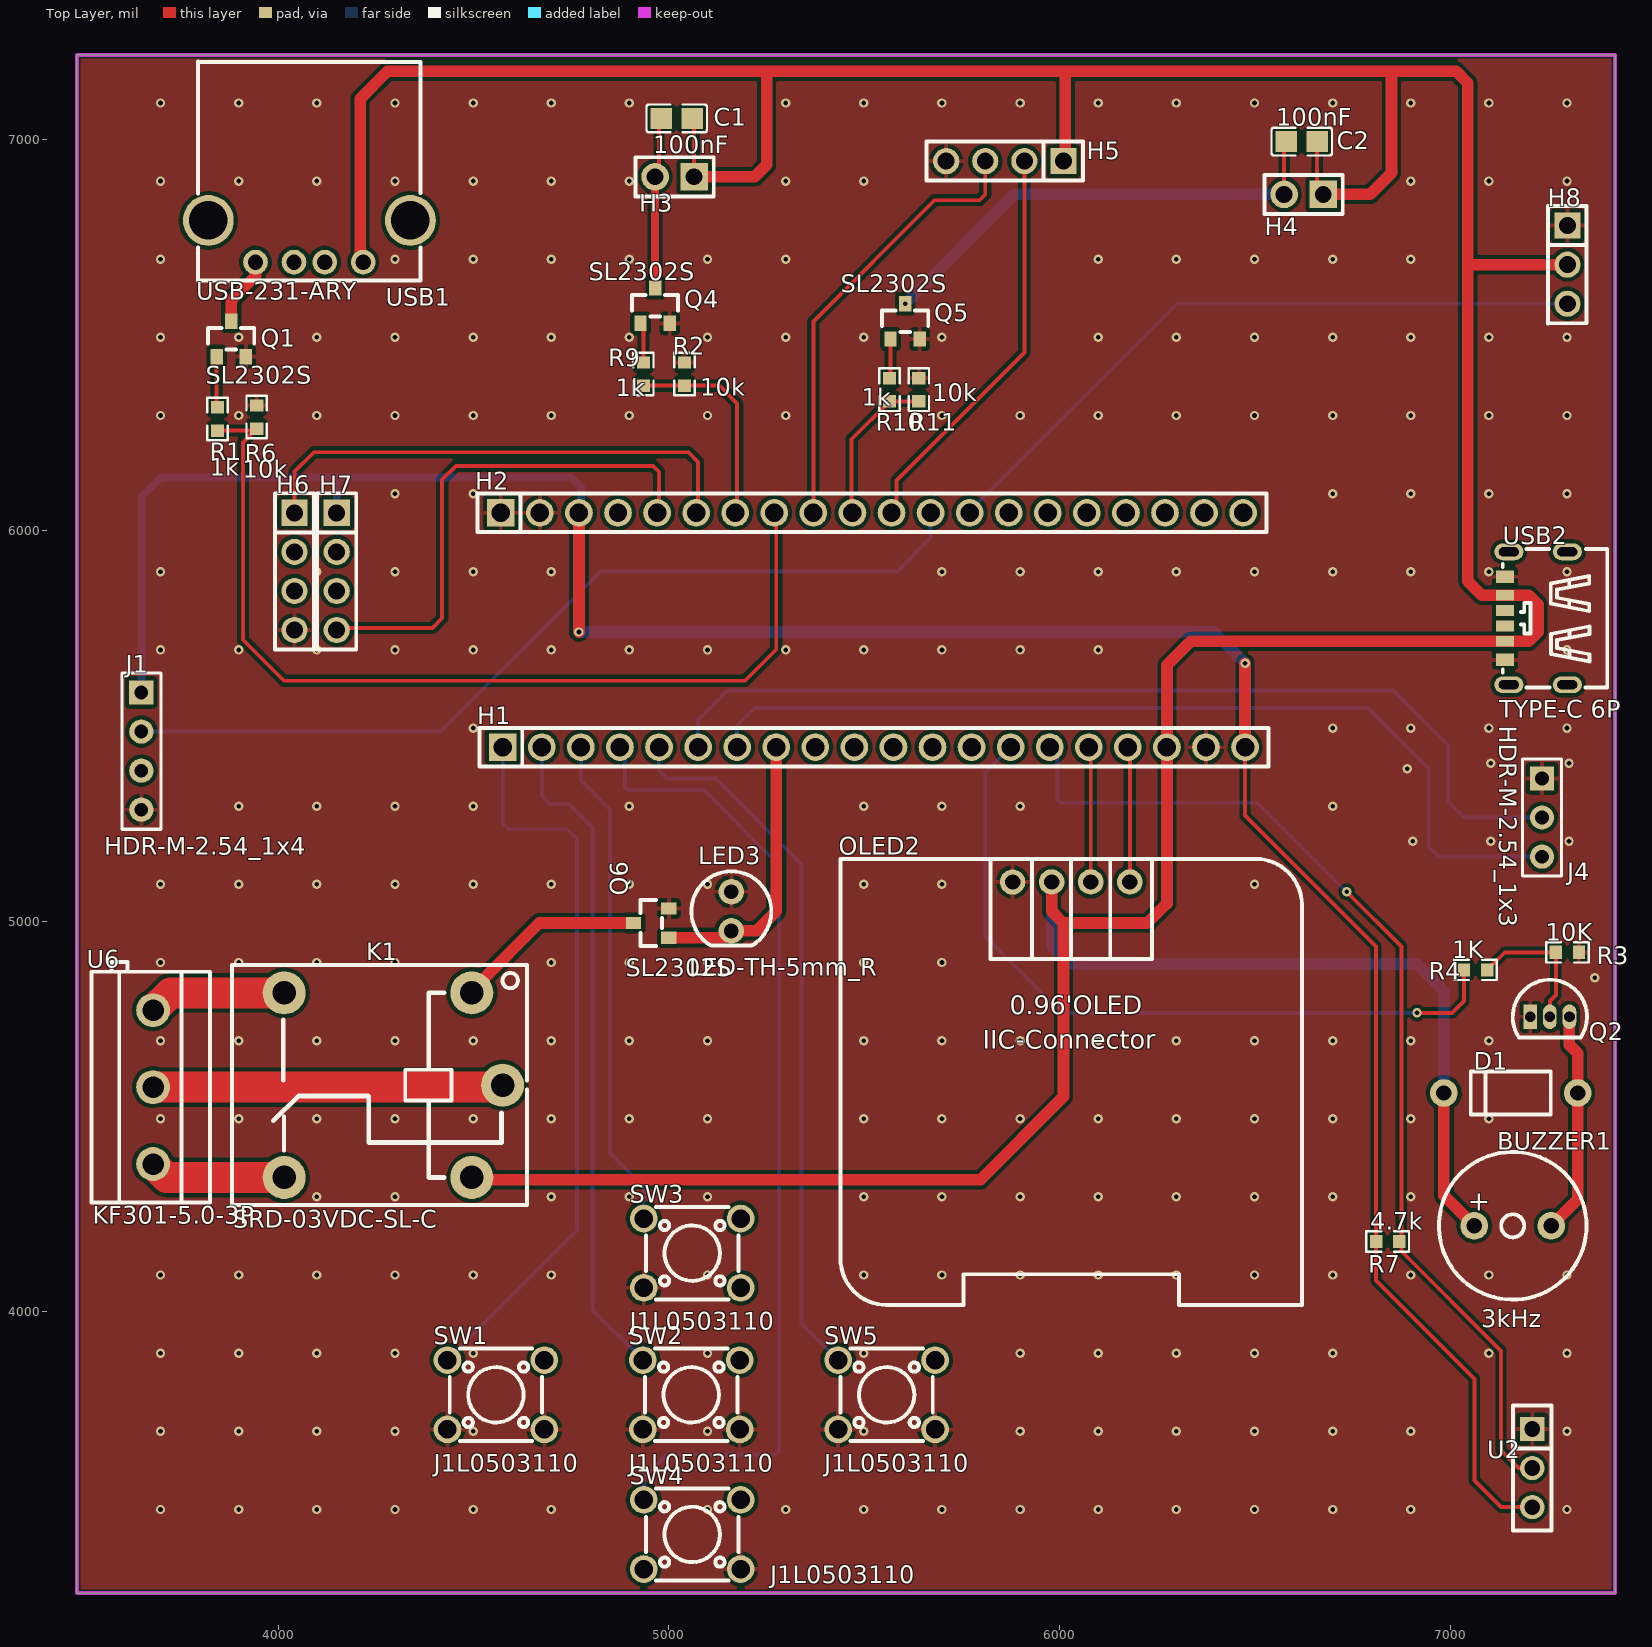
[diagram p0: Top Layer view]
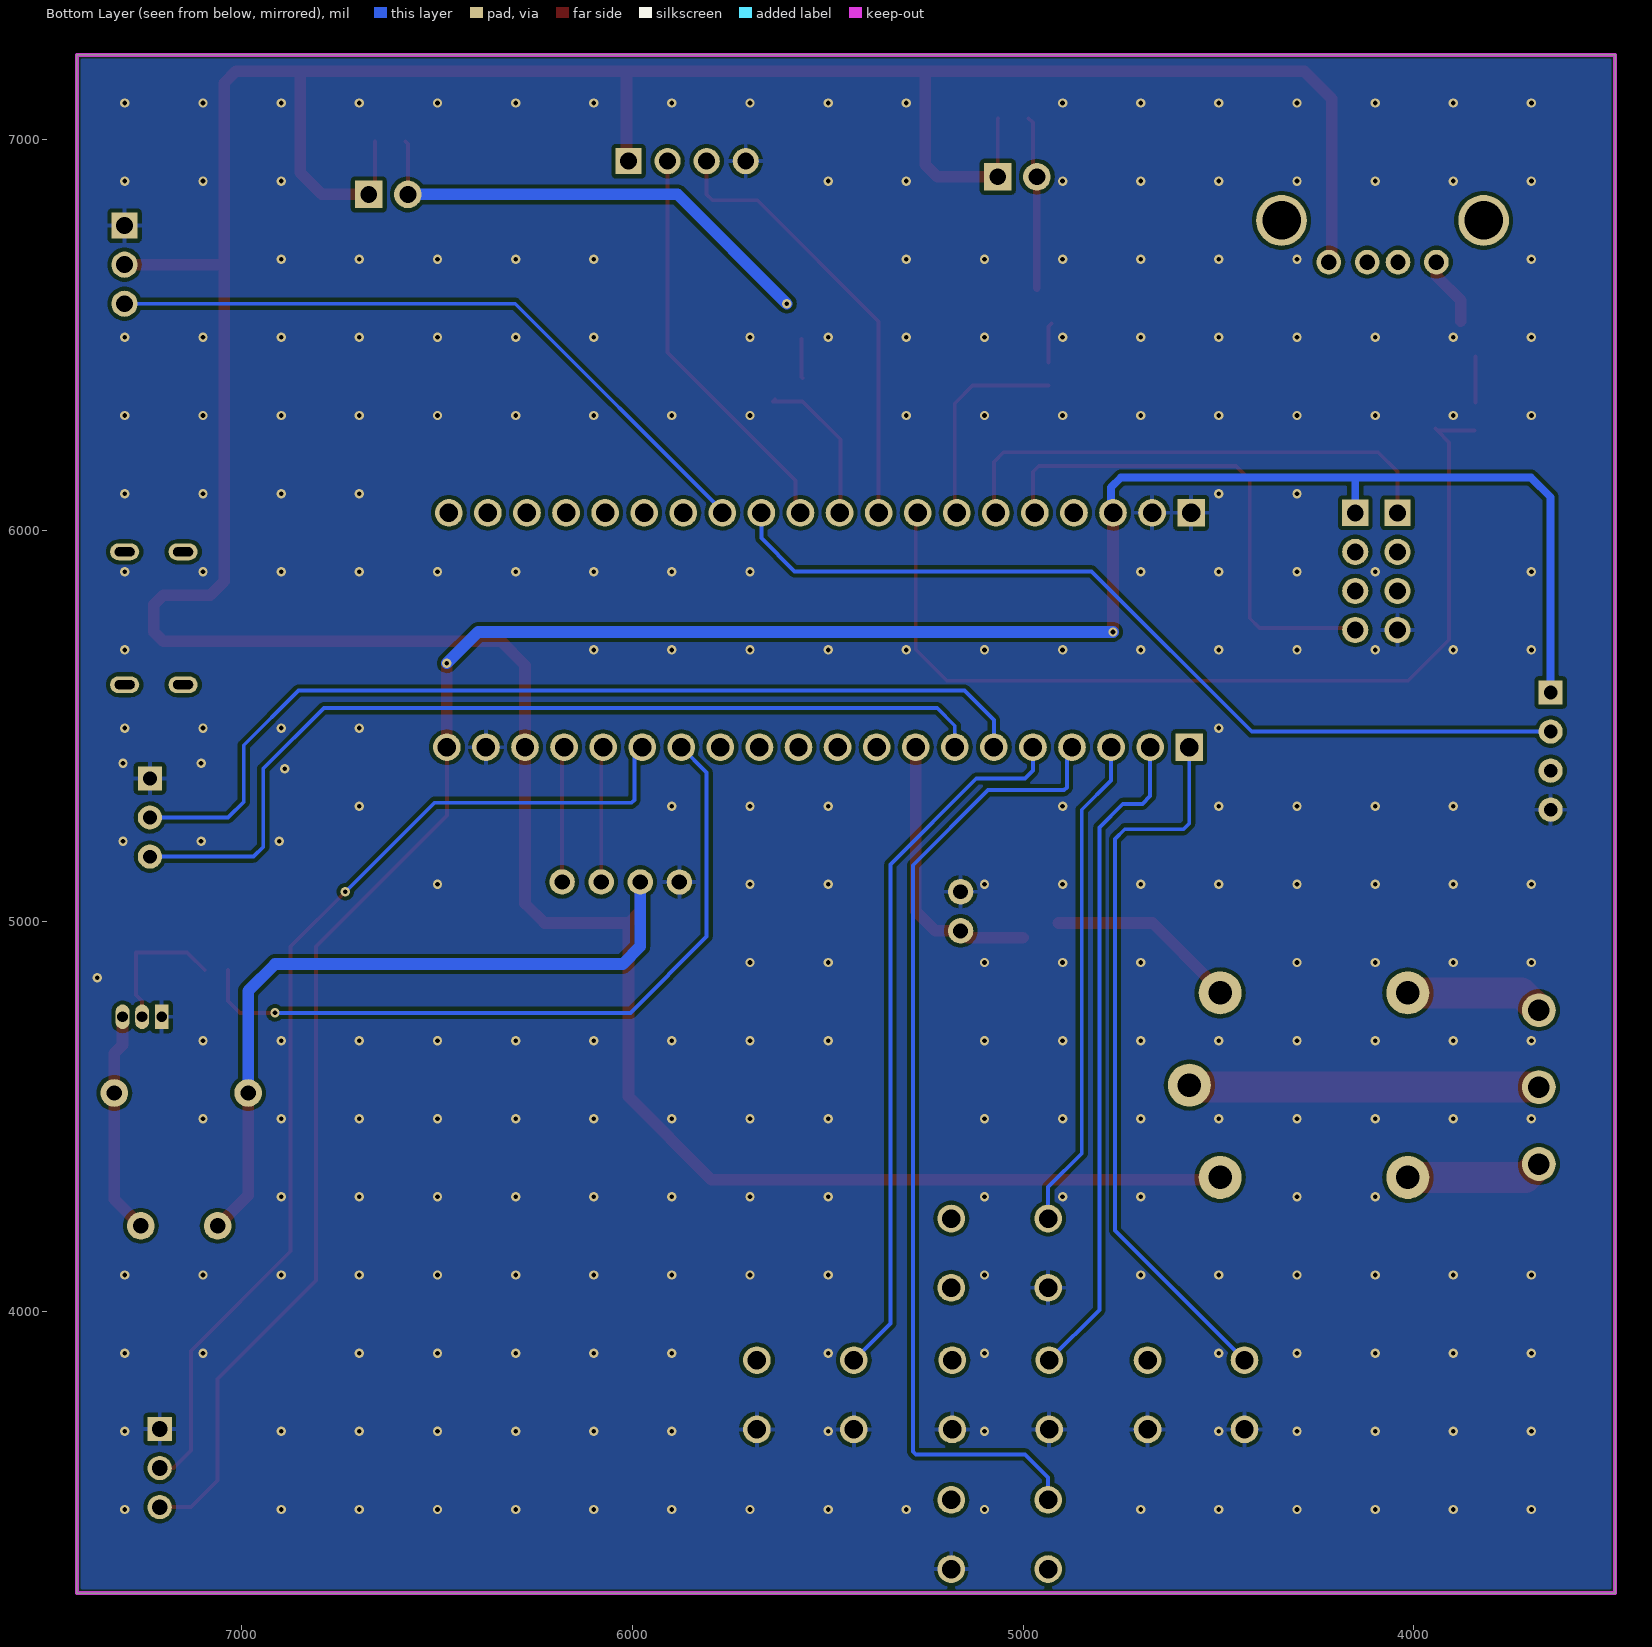
[diagram p1: Bottom Layer view, seen from below]
# Altium PCB MISC75408.pcbdoc
Units mil, origin at the board's own origin, x right, y up, seen from the top; angles counter-clockwise.
Board outline 3937 x 3937.11 mil, 2 copper layers (Top Layer, Bottom Layer), stack 62.206 mil thick; 40 components, 37 nets, 160 pads, 267 vias.

## Layer stack, top to bottom
Top Solder Mask Layer: solder mask 0.394, Dk 3.3
Top Layer: signal copper 1.379
Dielectric1: surface 59.449, FR4, Dk 4.5
Bottom Layer: signal copper 1.378
Bottom Solder Mask Layer: solder mask 0.394, Dk 3.3

## Board outline
3485,7217.01 3485,3279.9 7422,3279.9 7422,7217.01

## Design rules (kind name [scope] priority, off if disabled: settings)
BoardOutlineClearance copperThickness2oz_1 [All] p2 off: genericclearance=7.99 ignorepadtopadclearanceinfootprint=FALSE except(0: Arc-SplitContinuation Track-SplitContinuation SMDPad-SplitContinuation THPad-SplitContinuation Via-SplitContinuation Fill-SplitContinuation Region-SplitContinuation Poly-SplitContinuation Text-SplitContinuation Hole-SplitContinuation; 5.98: Arc-CutoutEdge SMDPad-CutoutEdge THPad-CutoutEdge Via-CutoutEdge Fill-CutoutEdge Region-CutoutEdge Text-CutoutEdge; 6.93: Hole-OutlineEdge Hole-CutoutEdge; 10: Poly-OutlineEdge Poly-CutoutEdge; 11.81: Arc-OutlineEdge Track-OutlineEdge SMDPad-OutlineEdge THPad-OutlineEdge Via-OutlineEdge Fill-OutlineEdge Region-OutlineEdge Text-OutlineEdge Track-CutoutEdge)
BoardOutlineClearance Plane_innerPlane_1 [All] p4 off: genericclearance=4.02 ignorepadtopadclearanceinfootprint=FALSE except(0: Arc-SplitContinuation Track-SplitContinuation SMDPad-SplitContinuation THPad-SplitContinuation Via-SplitContinuation Fill-SplitContinuation Region-SplitContinuation Poly-SplitContinuation Text-SplitContinuation Hole-SplitContinuation; 6: SMDPad-CutoutEdge THPad-CutoutEdge Via-CutoutEdge Fill-CutoutEdge Region-CutoutEdge Text-CutoutEdge; 6.93: Hole-OutlineEdge Hole-CutoutEdge; 10: Poly-OutlineEdge Poly-CutoutEdge; 11.8: Arc-OutlineEdge Track-OutlineEdge SMDPad-OutlineEdge THPad-OutlineEdge Via-OutlineEdge Fill-OutlineEdge Region-OutlineEdge Text-OutlineEdge; 11.81: Arc-CutoutEdge Track-CutoutEdge)
BoardOutlineClearance Copper_copperRegion_1 [All] p6 off: genericclearance=4.02 ignorepadtopadclearanceinfootprint=FALSE except(0: Arc-SplitContinuation Track-SplitContinuation SMDPad-SplitContinuation THPad-SplitContinuation Via-SplitContinuation Fill-SplitContinuation Region-SplitContinuation Poly-SplitContinuation Text-SplitContinuation Hole-SplitContinuation; 6: SMDPad-CutoutEdge THPad-CutoutEdge Via-CutoutEdge Fill-CutoutEdge Region-CutoutEdge Text-CutoutEdge; 6.93: Hole-OutlineEdge Hole-CutoutEdge; 10: Poly-OutlineEdge Poly-CutoutEdge; 11.8: Arc-OutlineEdge Track-OutlineEdge SMDPad-OutlineEdge THPad-OutlineEdge Via-OutlineEdge Fill-OutlineEdge Region-OutlineEdge Text-OutlineEdge; 11.81: Arc-CutoutEdge Track-CutoutEdge)
BoardOutlineClearance Copper_copperRegion_copperThickness1oz_1 [All] p8 off: genericclearance=4.02 ignorepadtopadclearanceinfootprint=FALSE except(0: Arc-SplitContinuation Track-SplitContinuation SMDPad-SplitContinuation THPad-SplitContinuation Via-SplitContinuation Fill-SplitContinuation Region-SplitContinuation Poly-SplitContinuation Text-SplitContinuation Hole-SplitContinuation; 6: SMDPad-CutoutEdge THPad-CutoutEdge Via-CutoutEdge Fill-CutoutEdge Region-CutoutEdge Text-CutoutEdge; 6.93: Hole-OutlineEdge Hole-CutoutEdge; 10: Poly-OutlineEdge Poly-CutoutEdge; 11.8: Arc-OutlineEdge Track-OutlineEdge SMDPad-OutlineEdge THPad-OutlineEdge Via-OutlineEdge Fill-OutlineEdge Region-OutlineEdge Text-OutlineEdge; 11.81: Arc-CutoutEdge Track-CutoutEdge)
BoardOutlineClearance Copper_copperRegion_Copper_copperRegion_1 [All] p10 off: genericclearance=4.02 ignorepadtopadclearanceinfootprint=FALSE except(0: Arc-SplitContinuation Track-SplitContinuation SMDPad-SplitContinuation THPad-SplitContinuation Via-SplitContinuation Fill-SplitContinuation Region-SplitContinuation Poly-SplitContinuation Text-SplitContinuation Hole-SplitContinuation; 6: SMDPad-CutoutEdge THPad-CutoutEdge Via-CutoutEdge Fill-CutoutEdge Region-CutoutEdge Text-CutoutEdge; 6.93: Hole-OutlineEdge Hole-CutoutEdge; 10: Poly-OutlineEdge Poly-CutoutEdge; 11.8: Arc-OutlineEdge Track-OutlineEdge SMDPad-OutlineEdge THPad-OutlineEdge Via-OutlineEdge Fill-OutlineEdge Region-OutlineEdge Text-OutlineEdge; 11.81: Arc-CutoutEdge Track-CutoutEdge)
BoardOutlineClearance copperThickness1oz_1 [All] p12: genericclearance=4.02 ignorepadtopadclearanceinfootprint=FALSE except(0: Arc-SplitContinuation Track-SplitContinuation SMDPad-SplitContinuation THPad-SplitContinuation Via-SplitContinuation Fill-SplitContinuation Region-SplitContinuation Poly-SplitContinuation Text-SplitContinuation Hole-SplitContinuation; 6: SMDPad-CutoutEdge THPad-CutoutEdge Via-CutoutEdge Fill-CutoutEdge Region-CutoutEdge Text-CutoutEdge; 6.93: Hole-OutlineEdge Hole-CutoutEdge; 10: Poly-OutlineEdge Poly-CutoutEdge; 11.8: Arc-OutlineEdge Track-OutlineEdge SMDPad-OutlineEdge THPad-OutlineEdge Via-OutlineEdge Fill-OutlineEdge Region-OutlineEdge Text-OutlineEdge; 11.81: Arc-CutoutEdge Track-CutoutEdge)
Clearance copperThickness2oz [All] p1 off: gap=7.99 ignorepadtopadclearanceinfootprint=FALSE except(5.98: SMDPad-Track SMDPad-SMDPad THPad-Track SMDPad-THPad THPad-THPad Track-Via SMDPad-Via THPad-Via Via-Via Fill-Track Region-Track Fill-SMDPad Region-SMDPad Fill-THPad Region-THPad Fill-Via Region-Via Fill-Fill Fill-Region Region-Region Arc-Track Arc-SMDPad Arc-THPad Arc-Via Fill-Arc Region-Arc Arc-Arc Text-Track SMDPad-Text Text-THPad Text-Via Fill-Text Region-Text Arc-Text Text-Text; 6.93: Hole-Track Hole-SMDPad Hole-THPad Hole-Via Fill-Hole Region-Hole Hole-Arc Hole-Text; 10: Poly-Track Poly-SMDPad Poly-THPad Poly-Via Poly-Fill Poly-Region Poly-Poly Poly-Arc Poly-Text Poly-Hole)
Clearance Plane_innerPlane [All] p3 off: gap=4.02 ignorepadtopadclearanceinfootprint=FALSE except(5.98: SMDPad-Track SMDPad-SMDPad THPad-Track SMDPad-THPad THPad-THPad Track-Via SMDPad-Via THPad-Via Via-Via Fill-Track Region-Track Fill-SMDPad Region-SMDPad Fill-THPad Region-THPad Fill-Via Region-Via Fill-Fill Fill-Region Region-Region; 6: Arc-Track Arc-SMDPad Arc-THPad Arc-Via Fill-Arc Region-Arc Arc-Arc Text-Track SMDPad-Text Text-THPad Text-Via Fill-Text Region-Text Arc-Text Text-Text; 6.93: Hole-Track Hole-SMDPad Hole-THPad Hole-Via Fill-Hole Region-Hole Hole-Arc Hole-Text; 10: Poly-Track Poly-SMDPad Poly-THPad Poly-Via Poly-Fill Poly-Region Poly-Poly Poly-Arc Poly-Text Poly-Hole)
Clearance Copper_copperRegion [All] p5 off: gap=4.02 ignorepadtopadclearanceinfootprint=FALSE except(5.98: SMDPad-Track SMDPad-SMDPad THPad-Track SMDPad-THPad THPad-THPad Track-Via SMDPad-Via THPad-Via Via-Via Fill-Track Region-Track Fill-SMDPad Region-SMDPad Fill-THPad Region-THPad Fill-Via Region-Via Fill-Fill Fill-Region Region-Region; 6: Arc-Track Arc-SMDPad Arc-THPad Arc-Via Fill-Arc Region-Arc Arc-Arc Text-Track SMDPad-Text Text-THPad Text-Via Fill-Text Region-Text Arc-Text Text-Text; 6.93: Hole-Track Hole-SMDPad Hole-THPad Hole-Via Fill-Hole Region-Hole Hole-Arc Hole-Text; 10: Poly-Track Poly-SMDPad Poly-THPad Poly-Via Poly-Fill Poly-Region Poly-Poly Poly-Arc Poly-Text Poly-Hole)
Clearance Copper_copperRegion_copperThickness1oz [All] p7 off: gap=4.02 ignorepadtopadclearanceinfootprint=FALSE except(5.98: SMDPad-Track SMDPad-SMDPad THPad-Track SMDPad-THPad THPad-THPad Track-Via SMDPad-Via THPad-Via Via-Via Fill-Track Region-Track Fill-SMDPad Region-SMDPad Fill-THPad Region-THPad Fill-Via Region-Via Fill-Fill Fill-Region Region-Region; 6: Arc-Track Arc-SMDPad Arc-THPad Arc-Via Fill-Arc Region-Arc Arc-Arc Text-Track SMDPad-Text Text-THPad Text-Via Fill-Text Region-Text Arc-Text Text-Text; 6.93: Hole-Track Hole-SMDPad Hole-THPad Hole-Via Fill-Hole Region-Hole Hole-Arc Hole-Text; 10: Poly-Track Poly-SMDPad Poly-THPad Poly-Via Poly-Fill Poly-Region Poly-Poly Poly-Arc Poly-Text Poly-Hole)
Clearance Copper_copperRegion_Copper_copperRegion [All] p9 off: gap=4.02 ignorepadtopadclearanceinfootprint=FALSE except(5.98: SMDPad-Track SMDPad-SMDPad THPad-Track SMDPad-THPad THPad-THPad Track-Via SMDPad-Via THPad-Via Via-Via Fill-Track Region-Track Fill-SMDPad Region-SMDPad Fill-THPad Region-THPad Fill-Via Region-Via Fill-Fill Fill-Region Region-Region; 6: Arc-Track Arc-SMDPad Arc-THPad Arc-Via Fill-Arc Region-Arc Arc-Arc Text-Track SMDPad-Text Text-THPad Text-Via Fill-Text Region-Text Arc-Text Text-Text; 6.93: Hole-Track Hole-SMDPad Hole-THPad Hole-Via Fill-Hole Region-Hole Hole-Arc Hole-Text; 10: Poly-Track Poly-SMDPad Poly-THPad Poly-Via Poly-Fill Poly-Region Poly-Poly Poly-Arc Poly-Text Poly-Hole)
Clearance copperThickness1oz [All] p11: gap=4.02 ignorepadtopadclearanceinfootprint=FALSE except(5.98: SMDPad-Track SMDPad-SMDPad THPad-Track SMDPad-THPad THPad-THPad Track-Via SMDPad-Via THPad-Via Via-Via Fill-Track Region-Track Fill-SMDPad Region-SMDPad Fill-THPad Region-THPad Fill-Via Region-Via Fill-Fill Fill-Region Region-Region; 6: Arc-Track Arc-SMDPad Arc-THPad Arc-Via Fill-Arc Region-Arc Arc-Arc Text-Track SMDPad-Text Text-THPad Text-Via Fill-Text Region-Text Arc-Text Text-Text; 6.93: Hole-Track Hole-SMDPad Hole-THPad Hole-Via Fill-Hole Region-Hole Hole-Arc Hole-Text; 10: Poly-Track Poly-SMDPad Poly-THPad Poly-Via Poly-Fill Poly-Region Poly-Poly Poly-Arc Poly-Text Poly-Hole)
DiffPairsRouting differentialPair [All] p1: maxlimit=6 minlimit=6 mostfreqgap=6 toplayer_minwidth=5 toplayer_prefwidth=10 toplayer_maxwidth=100 toplayer_mingap=6 toplayer_prefgap=6 toplayer_maxgap=6 bottomlayer_minwidth=5 bottomlayer_prefwidth=10 bottomlayer_maxwidth=100 bottomlayer_mingap=6 bottomlayer_prefgap=6 bottomlayer_maxgap=6 maxuncoupledlength=10
HoleToHoleClearance otherClearance [All] p1: gap=11.81 allowstackedmicrovias=TRUE
Length netLength [All] p1: minlimit=0 maxlimit=0
PasteMaskExpansion pasteMaskExpansion [All] p1: expansion=0
PlaneConnect innerPlane [All] p1: planeconnectstyle=Relief reliefexpansion=20 reliefentries=4 reliefconductorwidth=10 reliefairgap=10
PolygonConnect copperRegion_copperThickness1oz [All] p1 off: connectstyle=Relief reliefconductorwidth=10 reliefentries=4 polygonreliefangle="90 Angle" airgapwidth=10 via.connectstyle=Relief via.reliefconductorwidth=10 via.reliefentries=4 via.polygonreliefangle="90 Angle" via.airgapwidth=10
PolygonConnect copperRegion_Copper_copperRegion [All] p2 off: connectstyle=Relief reliefconductorwidth=10 reliefentries=4 polygonreliefangle="90 Angle" airgapwidth=10 via.connectstyle=Relief via.reliefconductorwidth=10 via.reliefentries=4 via.polygonreliefangle="90 Angle" via.airgapwidth=10
PolygonConnect copperRegion [All] p3: connectstyle=Relief reliefconductorwidth=10 reliefentries=4 polygonreliefangle="90 Angle" airgapwidth=10 via.connectstyle=Relief via.reliefconductorwidth=10 via.reliefentries=4 via.polygonreliefangle="90 Angle" via.airgapwidth=10
RoutingVias viaSize [All] p1: holewidth=12.01 width=24.02 viastyle="Through Hole" minholewidth=11.81 minwidth=19.68 maxholewidth=248.03 maxwidth=393.7
SolderMaskExpansion solderMaskExpansion [IsVia] p1: expansion=-1000 istentingtop=TRUE
SolderMaskExpansion solderMaskExpansion [All] p2: expansion=2 istentingtop=FALSE
Width copperThickness2oz_2 [All] p1 off: maxlimit=100 minlimit=8 preferedwidth=10
Width copperThickness1oz_2 [All] p2: maxlimit=100 minlimit=5 preferedwidth=10

## Components (designator, comment, footprint, x,y, rotation, side; value= is the part's Value field where it differs from the comment)
BUZZER1 "3kHz" BUZ-TH_BD9.6-P5.00-D0.7-FD 7160,4220 r0 top
C1 "100nF" C0805 5020.31,7054.47 r180 top
C2 "100nF" C0805 6620,6995 r180 top
D1 "" DO_1N4007 7155,4560 r0 top
H1 "" HDR-TH_20P-P2.54-V-F 5525,5445 r0 top
H2 "" HDR-TH_20P-P2.54-V-F 5520,6045 r0 top
H3 "" HDR-TH_2P-P2.54-V-M-1 5015,6905 r180 top
H4 "" HDR-TH_2P-P2.54-V-M-1 6625,6860 r180 top
H5 "" HDR-TH_4P-P2.54-V-M 5860,6945 r180 top
H6 "" HDR-TH_4P-P2.54-V-M 4041.84,5895 r270 top
H7 "" HDR-TH_4P-P2.54-V-M 4150,5895 r270 top
H8 "" HDR-TH_3P-P2.54-V-M 7300,6680 r270 top
J1 "HDR-M-2.54_1x4" HDR-M-2.54_1X4 3650,5435 r270 top
J4 "HDR-M-2.54_1x3" HDR-M-2.54_1X3 7235,5265 r270 top
K1 "SRD-03VDC-SL-C" RELAY-TH_SRD-XXVDC-XL-C 4295,4580 r180 top
LED3 "LED-TH-5mm_R" LED-TH_BD5.0_RED 5160,5025 r0 top
OLED2 "" 0.96OLED_4P 6030,5100 r0 top
Q1 "SL2302S" SOT-23_L2.9-W1.3-P1.90-LS2.4-BR 3880,6490 r270 top
Q2 "" S8050_TO_92 7255,4755 r0 top
Q4 "SL2302S" SOT-23_L2.9-W1.3-P1.90-LS2.4-BR 4965,6575 r270 top
Q5 "SL2302S" SOT-23_L2.9-W1.3-P1.90-LS2.4-BR 5605,6535 r270 top
Q6 "SL2302S" SOT-23_L2.9-W1.3-P1.90-LS2.4-BR 4955,4995 r0 top
R1 "1k" R0603 3845,6285 r90 top
R2 "10k" R0603 5040,6400 r90 top
R3 "10K" R0603 7300,4920 r180 top
R4 "1K" R0603 7065,4875 r180 top
R6 "10k" R0603 3945,6290 r90 top
R7 "4.7k" R0603 6840,4180 r180 top
R9 "1k" R0603 4935,6400 r90 top
R10 "1k" R0603 5565,6360 r90 top
R11 "10k" R0603 5640,6360 r90 top
SW1 "J1L0503110" SW-TH_4P-L6.0-W6.0-P4.50-LS6.3 4557.5,3787.5 r0 top
SW2 "J1L0503110" SW-TH_4P-L6.0-W6.0-P4.50-LS6.3 5057.5,3787.5 r0 top
SW3 "J1L0503110" SW-TH_4P-L6.0-W6.0-P4.50-LS6.3 5060,4150 r0 top
SW4 "J1L0503110" SW-TH_4P-L6.0-W6.0-P4.50-LS6.3 5060,3430 r0 top
SW5 "J1L0503110" SW-TH_4P-L6.0-W6.0-P4.50-LS6.3 5557.5,3787.5 r0 top
U2 "DS18B20+" HDR-TH_3P-P2.54-V-F 7210,3600 r270 top
U6 "KF301-5.0-3P" CONN-TH_3P-P5.00_KF301-5.0-3P 3680,4575 r90 top
USB1 "USB-231-ARY" USB-A-TH_USB-231-ARY 4080,6740 r180 top
USB2 "TYPE-C 6P" TYPE-C-SMD_TYPE-C-6P_1 7220,5775 r90 top

## Footprints (in the part's own frame and the unit in brackets; to place one, negate y for a bottom-side part, rotate by r counter-clockwise, add the part's x,y. Pads: shape width x height; smd on the part's side, far side on the other; paste and mask are expansions set on the pad)
0.96OLED_4P [mm]
  round 1.65 hole 1 copper offset 0,0: 1(-3.81,-0.001) 2(-1.27,0.002) 3(1.27,0.002) 4(3.81,0.002)
  silkscreen extent -15,-27.5 15,1.5
BUZ-TH_BD9.6-P5.00-D0.7-FD [mm]
  round 1.8 hole 1: 1(-2.5,0) 2(2.5,0)
  silkscreen extent -4.8,-4.8 4.8,4.8
C0805 [mm]
  rect 1.41x1.35 smd paste-100 mask+0.051: 1(-1,0) 2(1,0)
  silkscreen extent -1.96,-0.9 1.96,0.9
CONN-TH_3P-P5.00_KF301-5.0-3P [mm]
  round 2.2 hole 1.4 paste+0 mask+0.051: 1(-5,0) 2(0,0) 3(5,0)
  silkscreen extent -7.5,-3.7 8.13,4
DO_1N4007 [mm]
  round 1.8 hole 1 paste+0 mask+0.051: 1(-4.35,0) 2(4.35,0)
  silkscreen extent -2.6,-1.4 2.6,1.4
HDR-M-2.54_1X3 [mil]
  rect 62x62 hole 35 paste+0 mask+2: 1(-100,0)
  round 62 hole 35 paste+0 mask+2: 2(0,0) 3(100,0)
  silkscreen extent -150,-50 150,50
HDR-M-2.54_1X4 [mil]
  rect 62x62 hole 35 paste+0 mask+2: 1(-150,0)
  round 62 hole 35 paste+0 mask+2: 2(-50,0) 3(50,0) 4(150,0)
  silkscreen extent -200,-50 200,50
HDR-TH_2P-P2.54-V-M-1 [mm]
  rect 1.8x1.8 hole 1.1: 1(-1.27,0)
  round 1.8 hole 1.1: 2(1.27,0)
  silkscreen extent -2.54,-1.27 2.54,1.27
HDR-TH_3P-P2.54-V-F [mil]
  rect 62x62 hole 40.16: 1(-100,0)
  round 62 hole 40.16: 2(0,0) 3(100,0)
  silkscreen extent -160,-49 160,49
HDR-TH_3P-P2.54-V-M [mm]
  rect 1.7x1.7 hole 1.1: 1(-2.54,0)
  round 1.7 hole 1.1: 2(0,0) 3(2.54,0)
  silkscreen extent -3.81,-1.25 3.81,1.25
HDR-TH_4P-P2.54-V-M [mm]
  rect 1.7x1.7 hole 1.1: 1(-3.81,0)
  round 1.7 hole 1.1: 2(-1.27,0) 3(1.27,0) 4(3.81,0)
  silkscreen extent -5.08,-1.27 5.08,1.27
HDR-TH_20P-P2.54-V-F [mm]
  rect 1.8x1.8 hole 1.2: 1(-24.13,0)
  round 1.8 hole 1.2: 2(-21.59,0) 3(-19.05,0) 4(-16.51,0) 5(-13.97,0) 6(-11.43,0) 7(-8.89,0) 8(-6.35,0) 9(-3.81,0) 10(-1.27,0) 11(1.27,0) 12(3.81,0) 13(6.35,0) 14(8.89,0) 15(11.43,0) 16(13.97,0) 17(16.51,0) 18(19.05,0) 19(21.59,0) 20(24.13,0)
  silkscreen extent -25.65,-1.25 25.65,1.25
LED-TH_BD5.0_RED [mil]
  round 65 hole 38 paste+0 mask+2: 1(0,50) 2(0,-50)
  silkscreen extent -102,-88 102,102
R0603 [mil]
  rect 31.75x34.02 smd paste-3937.01 mask+2: 1(-29.66,-0.01) 2(29.66,0.01)
  silkscreen extent -55,-26 55,26
RELAY-TH_SRD-XXVDC-XL-C [mil]
  round 110 hole 60 paste+0 mask+2: 1(-200.79,-236.22) 2(279.53,-236.2) 3(279.53,236.2) 4(-200.79,236.22) 5(-279.53,0)
  silkscreen extent -342,-307 413,307
S8050_TO_92 [mil]
  rect 35.4x63 hole 27.6 paste+0 mask+2: 1(-50,0)
  oval 35.4x63 hole 27.6 paste+0 mask+2: 2(0,0) 3(50,0)
  silkscreen extent -95,-53 95,95
SOT-23_L2.9-W1.3-P1.90-LS2.4-BR [mm]
  rect 1x0.8 smd paste+0 mask+0.051: 1(1.15,-0.95) 2(1.15,0.95) 3(-1.15,0)
  silkscreen extent -0.7,-1.5 0.7,1.5
SW-TH_4P-L6.0-W6.0-P4.50-LS6.3 [mm]
  round 1.8 hole 1.2: 1(-3.15,2.25) 2(3.15,2.25) 3(-3.15,-2.25) 4(3.15,-2.25)
  silkscreen extent -3,-3 3,3
TYPE-C-SMD_TYPE-C-6P_1 [mm]
  oval 1.1x1.9 hole 0.6 slot 1.3 at 90 deg paste+0 mask+0.051: 7(-4.32,1.775) 7(-4.32,-2.025) 7(4.32,1.775)
  oval 1.1x1.9 hole 0.6 slot 1.3 at 90 deg copper offset 0,0 paste+0 mask+0.051: 7(4.32,-2.025)
  rect 0.7x1.2 smd paste-100 mask+0.051: A5(-0.5,2.025) A9(1.5,2.025) B5(0.5,2.025) B9(-1.5,2.025)
  rect 0.8x1.2 smd paste-100 mask+0.051: A12(2.7,2.025) B12(-2.7,2.025)
  silkscreen extent -4.5,-4.63 4.5,2.18
USB-A-TH_USB-231-ARY [mm]
  round 1.6 hole 1: 1(-3.5,1.355) 2(-1,1.355) 3(1,1.355) 4(3.5,1.355)
  round 3.3 hole 2.5: 5(-6.57,-1.355) 6(6.57,-1.355)
  silkscreen extent -7.23,-11.68 7.24,2.54

## Via types
v1: diameter 24.02, hole 12, Top Layer to Bottom Layer, 267 vias

## Nets (pads, with @x,y where several pads share a name; then routed paths per layer and width w, separated by ;. In a path a pad name is that pad's centre, name@x,y a point inside that pad or via, vN(x,y) a via of type N, cw(c..) or ccw(c..) an arc to the next point about the centre after c; other vN are vias at no path point)
$1N2: Q1.3 USB1.4 | length 177.2
  Top Layer w30: Q1.3 3880,6588.86 3942.21,6651.07 USB1.4
$1N4: Q1.1 R1.2 | length 117
  Top Layer w10: R1.2@3842.6,6327.74 Q1.1
$1N10: BUZZER1.2 D1.2 Q2.3 | length 571.9
  Top Layer w30: BUZZER1.2 7326.26,4287.84 D1.2 7326.26,4661.65 7305,4682.91 Q2.3
$1N26: Q4.1 R9.2 | length 103.1
  Top Layer w10: Q4.1 4935,6522.32 R9.2
$1N27: C1.2 H3.2 Q4.3 | length 442.9
  Top Layer w10: H3.2 4975,6915 4975,7043.54 C1.2@4985.94,7054.47
  Top Layer w20: Q4.3 H3.2
$1N30: C2.2 H4.2 Q5.3 | length 1223.2
  Top Layer w10: H4.2 6575,6989.37 C2.2
  Bottom Layer w30: v1(5605,6580.27) 5884.73,6860 H4.2
$1N32: Q5.1 R10.2 | length 101.1
  Top Layer w10: R10.2 5567.6,6392.26 Q5.1
$1N35: K1.2 U6.3 | length 353.8
  Top Layer w80: U6.3 3724.35,4816.2 K1.2
$1N38: K1.5 U6.2 | length 896.6
  Top Layer w80: U6.2 4569.53,4575 K1.5
$1N39: K1.3 U6.1 | length 349.7
  Top Layer w80: U6.1 3714.35,4343.8 K1.3
$1N121: K1.1 Q6.3 | length 457.1
  Top Layer w30: K1.1@4515.89,4842.23 4668.66,4995 Q6.3
$1N124: Q2.2 R3.2 R4.1 | length 365.7
  Top Layer w10: R4.1 7139.66,4920 R3.2 7270.34,4810.34 7255,4795 Q2.2
+5V: BUZZER1.1 C1.1 C2.1 D1.1 H1.18 H3.1 H4.1 H5.1 H8.2 K1.4 OLED2.2 USB1.1 USB2.A9 USB2.B9 | length 12373.8
  Top Layer w10: C1.1@5064.68,7054.47 5065,7054.15 H3.1 ; C2.1 6659.37,6875.63 H4.1
  Top Layer w30: USB1.1 4210,6694.45 4210,7105 4280,7175 5250.56,7175 ; K1.4@4528.61,4337.87 5797.87,4337.87 6010,4550 6010,4995 ; H3.1 5220,6905 5250.56,6935.56 5250.56,7175 ; OLED2.2@5980,5100.05 5980,5025 6010,4995 ; H5.1@6015,6955 6015,7175 ; H4.1 6795,6860 6850,6915 6850,7173.29 6851.71,7175 ; D1.1 6983.74,4297.84 BUZZER1.1 ; H8.2 7049.06,6680 7045,6675.94 ; 5250.56,7175 6015,7175 ; 6010,4995 6225,4995 6275,5045 H1.18 6275,5655 6335.95,5715.95 7140.27,5715.95 7200.95,5715.95 7225,5740 7225,5810 7200.94,5834.06 USB2.A9 7080.94,5834.06 7045,5870 7045,6675.94 ; 6015,7175 6851.71,7175 ; 6851.71,7175 7015,7175 7045,7145 7045,6675.94
  Bottom Layer w30: OLED2.2@5980,5100.05 5980,4935 6025,4890 6915,4890 6983.74,4821.26 D1.1
GND: H1.19 H2.1 H2.2 H5.4 H6.4 H8.1 J1.4 J4.1 LED3.1 OLED2.1 Q1.2 Q2.1 Q4.2 Q5.2 Q6.2 R2.2 R3.1 R6.2 R11.2 SW1.3 SW1.4 SW2.3 SW2.4 SW3.3 SW4.4 SW5.3 SW5.4 U2.1 USB2.A12 USB2.B12
  other v1: 3699.1,3494 3899.1,3494 4099.1,3494 4299.1,3494 4499.1,3494 4699.1,3494 5099.1,3494 5299.1,3494 5499.1,3494 5699.1,3494 5899.1,3494 6099.1,3494 6299.1,3494 6499.1,3494 6699.1,3494 6899.1,3494 7299.1,3494 3699.1,3694 3899.1,3694 4099.1,3694 4299.1,3694 4499.1,3694 5099.1,3694 5499.1,3694 5899.1,3694 6099.1,3694 6299.1,3694 6499.1,3694 6699.1,3694 6899.1,3694 7299.1,3694 3699.1,3894 3899.1,3894 4099.1,3894 4299.1,3894 4499.1,3894 5099.1,3894 5499.1,3894 5899.1,3894 6099.1,3894 6299.1,3894 6499.1,3894 6699.1,3894 7099.1,3894 7299.1,3894 3699.1,4094 3899.1,4094 4099.1,4094 4299.1,4094 4499.1,4094 4699.1,4094 5099.1,4094 5499.1,4094 5699.1,4094 5899.1,4094 6099.1,4094 6299.1,4094 6499.1,4094 6699.1,4094 6899.1,4094 7099.1,4094 7299.1,4094 4099.1,4294 4299.1,4294 4699.1,4294 4899.1,4294 5099.1,4294 5499.1,4294 5699.1,4294 5899.1,4294 6099.1,4294 6299.1,4294 6499.1,4294 6699.1,4294 6899.1,4294 3699.1,4494 3899.1,4494 4099.1,4494 4299.1,4494 4499.1,4494 4699.1,4494 4899.1,4494 5099.1,4494 5499.1,4494 5699.1,4494 5899.1,4494 6099.1,4494 6299.1,4494 6499.1,4494 6699.1,4494 6899.1,4494 7099.1,4494 3699.1,4694 3899.1,4694 4099.1,4694 4299.1,4694 4499.1,4694 4699.1,4694 4899.1,4694 5099.1,4694 5499.1,4694 5699.1,4694 5899.1,4694 6099.1,4694 6299.1,4694 6499.1,4694 6699.1,4694 6899.1,4694 7099.1,4694 7370,4855 3699.1,4894 3899.1,4894 4099.1,4894 4299.1,4894 4699.1,4894 4899.1,4894 5099.1,4894 5499.1,4894 5699.1,4894 3699.1,5094 3899.1,5094 4099.1,5094 4299.1,5094 4499.1,5094 4699.1,5094 4899.1,5094 5099.1,5094 5499.1,5094 5699.1,5094 6499.1,5094 6904.1,5204 7104.1,5204 7304.1,5204 3899.1,5294 4099.1,5294 4299.1,5294 4499.1,5294 4899.1,5294 5499.1,5294 5699.1,5294 5899.1,5294 6699.1,5294 6890,5390 7104.1,5404 7304.1,5404 4499.1,5494 6699.1,5494 6899.1,5494 7099.1,5494 7299.1,5494 3699.1,5694 3899.1,5694 4099.1,5694 4299.1,5694 4499.1,5694 4699.1,5694 4899.1,5694 5099.1,5694 5299.1,5694 5499.1,5694 5699.1,5694 5899.1,5694 6099.1,5694 7299.1,5694 3699.1,5894 4099.1,5894 4299.1,5894 4499.1,5894 4699.1,5894 5699.1,5894 5899.1,5894 6099.1,5894 6299.1,5894 6499.1,5894 6699.1,5894 6899.1,5894 7099.1,5894 7299.1,5894 4299.1,6094 4499.1,6094 6699.1,6094 6899.1,6094 7099.1,6094 7299.1,6094 3699.1,6294 3899.1,6294 4099.1,6294 4299.1,6294 4499.1,6294 4699.1,6294 4899.1,6294 5099.1,6294 5299.1,6294 5699.1,6294 5899.1,6294 6099.1,6294 6299.1,6294 6499.1,6294 6699.1,6294 6899.1,6294 7099.1,6294 7299.1,6294 3699.1,6494 3899.1,6494 4099.1,6494 4299.1,6494 4499.1,6494 4699.1,6494 4899.1,6494 5099.1,6494 5299.1,6494 5499.1,6494 5699.1,6494 6099.1,6494 6299.1,6494 6499.1,6494 6699.1,6494 6899.1,6494 7099.1,6494 7299.1,6494 3699.1,6694 4299.1,6694 4499.1,6694 4699.1,6694 4899.1,6694 5099.1,6694 5299.1,6694 6099.1,6694 6299.1,6694 6499.1,6694 6699.1,6694 6899.1,6694 3699.1,6894 3899.1,6894 4099.1,6894 4299.1,6894 4499.1,6894 4699.1,6894 4899.1,6894 5299.1,6894 5499.1,6894 6899.1,6894 7099.1,6894 7299.1,6894 3699.1,7094 3899.1,7094 4099.1,7094 4299.1,7094 4499.1,7094 4699.1,7094 4899.1,7094 5299.1,7094 5499.1,7094 5699.1,7094 5899.1,7094 6099.1,7094 6299.1,7094 6499.1,7094 6699.1,7094 6899.1,7094 7099.1,7094 7299.1,7094
PA3: H2.13 H8.3 | length 1754.5
  Bottom Layer w10: H2.13 5770,6050 6300,6580 H8.3
PA4: H2.12 J1.2 | length 2290
  Bottom Layer w10: J1.2 4415,5485 4825,5895 5585,5895 5670,5980 H2.12
PA5: H2.11 H5.2 | length 1040.8
  Top Layer w10: H2.11 5582.93,6057.93 5582.93,6127.93 5910,6455 H5.2
PA6: H2.10 R10.1 R11.1 | length 410.5
  Top Layer w10: H2.10@5475,6045 5467.93,6052.07 5467.93,6233.27 R10.1 R11.1@5630,6330.34 ; R11.1@5635,6335.34 R11.1@5630,6330.34 ; R11.1 R11.1@5630,6330.34
PA7: H2.9 H5.3 | length 1149.6
  Top Layer w10: H2.9 5370,6535 5680,6845 5795,6845 5810,6860 H5.3
PA8: H1.5 SW5.1 | length 1832.1
  Bottom Layer w10: H1.5 4975,5385 4995,5365 5120,5365 5340,5145 5340,3969.56 SW5.1
PA9: H1.6 J4.2 | length 2480.6
  Bottom Layer w10: H1.6 5075,5515 5150,5590 6855,5590 6995,5450 6995,5305 7035,5265 J4.2
PA10: H1.7 J4.3 | length 2408.2
  Bottom Layer w10: H1.7 5175,5500 5220,5545 6790,5545 6945,5390 6945,5190 6970,5165 J4.3
PA11: H1.8 LED3.2 Q6.1 | length 722.6
  Top Layer w30: Q6.1 5142.6,4957.6 LED3.2 5225,4975 5275,5025 H1.8
PB0: H2.8 R1.1 R6.1 | length 2441.5
  Top Layer w10: R1.1 R6.1@3940,6255.34 ; R6.1 R6.1@3940,6255.34 ; H2.8@5275,6045 5275,5695 5195,5615 4015,5615 3910,5720 3910,6225.34 R6.1@3940,6255.34
PB1: H2.7 R2.1 R9.1 | length 533.4
  Top Layer w10: R9.1 R2.1 5129.66,6370.34 5175,6325 H2.7@5175,6050.34
PB5: H1.13
PB6: H1.14 R4.2 | length 1910.3
  Top Layer w10: v1(6915,4765) 7005,4765 7035.34,4795.34 R4.2
  Bottom Layer w10: H1.14 5810,5380 5810,4960 6005,4765 v1(6915,4765)
PB7: H1.15 R7.1 U2.2 | length 2672.9
  Top Layer w10: v1(6735,5075) 6875,4935 6875,4154.8 7130,3899.8 7130,3645 7175,3600 U2.2
  Bottom Layer w10: H1.15 5995,5425 5995,5310 6002.07,5302.93 6507.07,5302.93 v1(6735,5075)
PB8: H1.16 OLED2.3 | length 347
  Top Layer w10: H1.16 6080,5440 OLED2.3@6080,5100.05
PB9: H1.17 OLED2.4 | length 347
  Top Layer w10: H1.17 6180,5440 OLED2.4@6180,5100.05
PB10: H2.6 H6.1 | length 1279.5
  Top Layer w10: H6.1@4041.84,6050 4041.84,6150.46 4091.38,6200 5050,6200 5075,6175 H2.6@5075,6060
PB11: H2.5 H7.4 | length 1316.1
  Top Layer w10: H7.4@4150,5750 4395,5750 4420,5775 4420,6130 4455,6165 4960,6165 4975,6150 H2.5@4975,6045
PB12: H1.1 SW1.1 | length 1872.8
  Bottom Layer w10: SW1.1 4765,4207.6 4765,5210 4740,5235 4590,5235 4575,5250 H1.1
PB13: H1.2 SW2.1 | length 1705.3
  Bottom Layer w10: H1.2 4675,5320 4695,5300 4745,5300 4805,5240 4805,4004.56 SW2.1
PB14: H1.3 SW3.1 | length 1273.1
  Bottom Layer w10: H1.3 4775,5360 4850,5285 4850,4405 4935.98,4319.02 SW3.1
PB15: H1.4 SW4.1 | length 2516.6
  Bottom Layer w10: H1.4 4887.93,5432.07 4887.93,5342.07 4895,5335 5090,5335 5282.07,5142.93 5282.07,3642.07 5275,3635 4995,3635 4935.98,3575.98 SW4.1
VCC: H1.20 H2.3 H7.1 J1.1 R7.2 U2.3 | length 6380.4
  Top Layer w10: H1.20 6475,5270 6810,4935 6810,4080 7061.78,3828.22 7061.78,3568.22 7130,3500 U2.3
  Top Layer w30: v1(4770,5740) H2.3 ; H1.20 v1(6475,5660)
  Bottom Layer w20: J1.1 3650,6085 3700,6135 4151.9,6135 ; H7.1 4150,6130 4151.9,6131.9 4151.9,6135 ; H2.3@4785,6035 4775,6045 4775,6110 4750,6135 4151.9,6135
  Bottom Layer w30: v1(4770,5740) 6395,5740 v1(6475,5660)
pads on no net: H1.9 H1.10 H1.11 H1.12 H2.4 H2.14 H2.15 H2.16 H2.17 H2.18 H2.19 H2.20 H6.2 H6.3 H7.2 H7.3 J1.3 SW1.2 SW2.2 SW3.2 SW3.4 SW4.2 SW4.3 SW5.2 USB1.2 USB1.3 USB1.5 USB1.6 USB2.7 USB2.A5 USB2.B5

## Polygon pours and split planes (outlines as drawn)
GND on Top Layer (solid, remove dead copper, pour order 0): 3000,7465 3000,3000 7905,3000 7905,7465
GND on Bottom Layer (solid, remove dead copper, pour order 2): 3315,7425 3315,3055 7620,3055 7620,7425

## Keep-outs
Board Outline Layer:
  the board outline again, w10